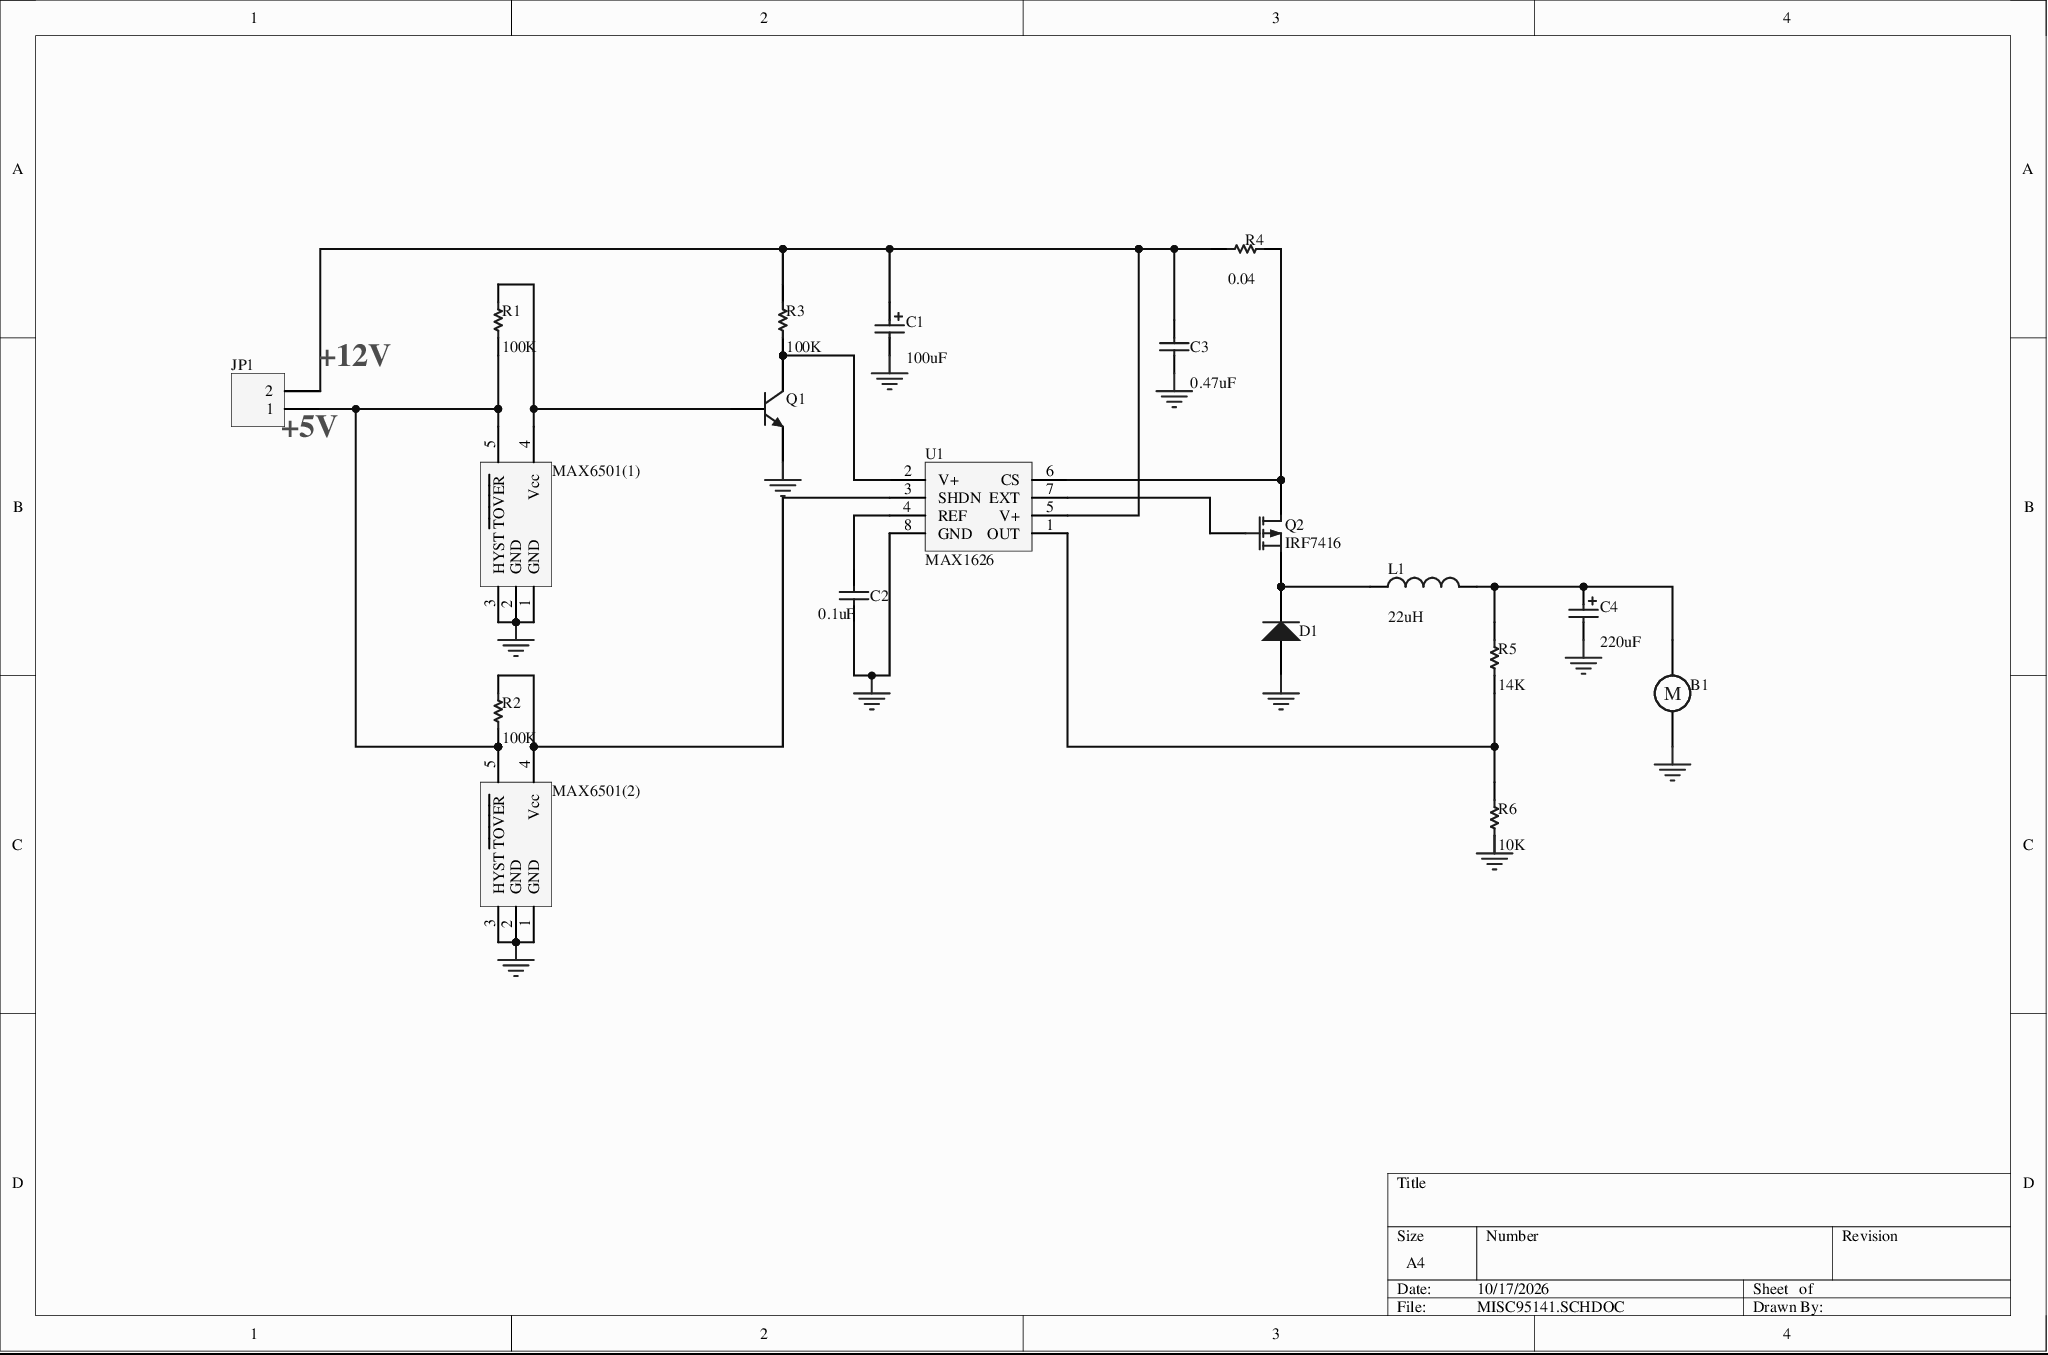
[diagram p0: MISC95141.SCHDOC]
# Altium project MISC95141.PRJPCB
1 sheet, 19 parts. Net scope: global (net labels, ports and power ports of the same name join across sheets).
Board file: MISC95141.PCBDOC

## Sheet MISC95141.SCHDOC
size A4

### Parts
B1  Motor  [RB5-10.5]  (value not drawn)
C1  value 100uF  [RB7.6-15]  (hidden comment: Cap Pol1)
C2  value 0.1uF  [RAD-0.3]  (hidden comment: Cap)
C3  value 0.47uF  [RAD-0.3]  (hidden comment: Cap)
C4  value 220uF  [RB7.6-15]  (hidden comment: Cap Pol1)
D1  Diode  [DSO-C2/X3.3]  (value not drawn)
JP1  Header 2  [HDR1X2]  (value not drawn)
L1  value 22uH  [CC4532-1812]  (hidden comment: Inductor)
MAX6501(1)  MAX6501  [SO-G5/P.95]  (value not drawn)
MAX6501(2)  MAX6501  [SO-G5/P.95]  (value not drawn)
Q1  NPN  [BCY-W3]  (value not drawn)
Q2  IRF7416  [BCY-W3/H.8]
R1  value 100K  [AXIAL-0.3]  (hidden comment: Res1)
R2  value 100K  [AXIAL-0.3]  (hidden comment: Res1)
R3  value 100K  [AXIAL-0.3]  (hidden comment: Res1)
R4  value 0.04  [AXIAL-0.3]  (hidden comment: Res1)
R5  value 14K  [AXIAL-0.3]  (hidden comment: Res1)
R6  value 10K  [AXIAL-0.3]  (hidden comment: Res1)
U1  MAX1626  [DIP-4]

### Nets
GND: B1.2 C1.2 C2.1 C3.1 C4.2 D1.1(A) MAX6501(1).1(GND) MAX6501(1).2(GND) MAX6501(1).3(HYST) MAX6501(2).1(GND) MAX6501(2).2(GND) MAX6501(2).3(HYST) Q1.3(E) U1.8(GND)
NetB1_1: B1.1 C4.1 L1.2 R5.2
NetC1_1: C1.1 C3.2 JP1.2 R3.2 R4.1 U1.5(V+)
NetC2_2: C2.2 U1.4(REF)
NetD1_2: D1.2(K) L1.1 Q2.3(S)
NetJP1_1: JP1.1 MAX6501(1).5(~{TOVER}) MAX6501(2).5(~{TOVER}) R1.1 R2.1
NetMAX6501(1)_4: MAX6501(1).4(Vcc) Q1.2(B) R1.2
NetMAX6501(2)_4: MAX6501(2).4(Vcc) R2.2 U1.3(SHDN)
NetQ1_1: Q1.1(C) R3.1 U1.2(V+)
NetQ2_1: Q2.1(D) R4.2 U1.6(CS)
NetQ2_2: Q2.2(G) U1.7(EXT)
NetR5_1: R5.1 R6.2 U1.1(OUT)

Not connected (* = marked no-connect by the designer): R6 1

### Notes on the sheet
- (near JP1) +12V
- (near JP1) +5V
- Labels drawn without touching a wire or pin: GND

### Library data of the parts
B1 = Motor: Motor, General Kind; Published: 24-Mar-1999; Revision: July-2002: Re-released for DXP Platform.; Publisher: COMPANY_A
C1 C4 = Cap Pol1: Polarized Capacitor (Radial); Published: 8-Jun-2000; Revision: July-2002: Re-released for DXP Platform.; Publisher: COMPANY_A
C2 C3 = Cap: Capacitor; Published: 8-Jun-2000; Revision: July-2002: Re-released for DXP Platform.; Publisher: COMPANY_A
D1 = Diode: Default Diode; Code - JEDEC: DO-214-AB; Published: 8-Jun-2000; Revision: July-2002: Re-released for DXP Platform.; Publisher: COMPANY_A
JP1 = Header 2: Header, 2-Pin; Revision: 17-Jul-2002: Re-released for DXP Platform.; Publisher: COMPANY_A
Q1 = NPN: NPN Bipolar Transistor; Code - JEDEC: TO-226-AA; Published: 8-Jun-2000; Revision: July-2002: Re-released for DXP Platform.; Publisher: COMPANY_A
Q2 = MOSFET-P: P-Channel MOSFET; Published: 8-Jun-2000; Revision: July-2002: Re-released for DXP Platform.; Publisher: COMPANY_A
R1-R6 = Res1: Resistor; Published: 8-Jun-2000; Revision: July-2002: Re-released for DXP Platform.; Publisher: COMPANY_A
L1 = Inductor: Published: 8-Jun-2000; Revision: July-2002: Re-released for DXP Platform.; Publisher: COMPANY_A